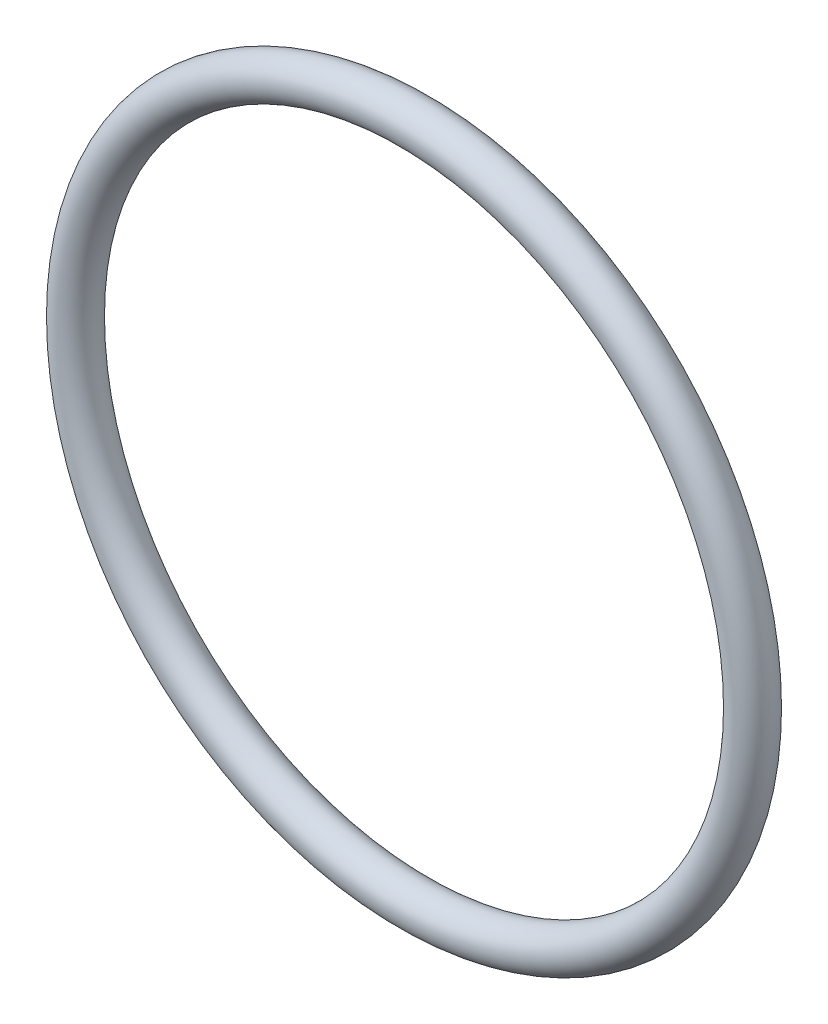
SolidWorks part; units mm, degrees
material "BUTYL"
ref_plane "Front Plane" through (0, 0, 0) normal (0, 0, 1) x (1, 0, 0)
ref_plane "Top Plane" through (0, 0, 0) normal (0, 1, 0) x (1, 0, 0)
ref_plane "Right Plane" through (0, 0, 0) normal (1, 0, 0) x (0, 0, -1)
sketch "Sketch1" plane through (0, 0, 0) normal (0, 0, 1) x (1, 0, 0)
  circle A0 centre (0, 0) radius 8.25
sketch "Sketch2" plane through (0, 0, 0) normal (0, 1, 0) x (1, 0, 0)
  line L0 (-8.25, 0) -> (8.25, 0) construction
  circle A0 centre (-8.25, 0) radius 0.5
sweep "Sweep1" add profiles "Sketch2" path "Sketch1"
sketch "Sketch3" plane through (0, 0, 0) normal (1, 0, 0) x (0, 0, -1)
  line L0 (2.4954, 0) -> (-3.1846, 0) construction
